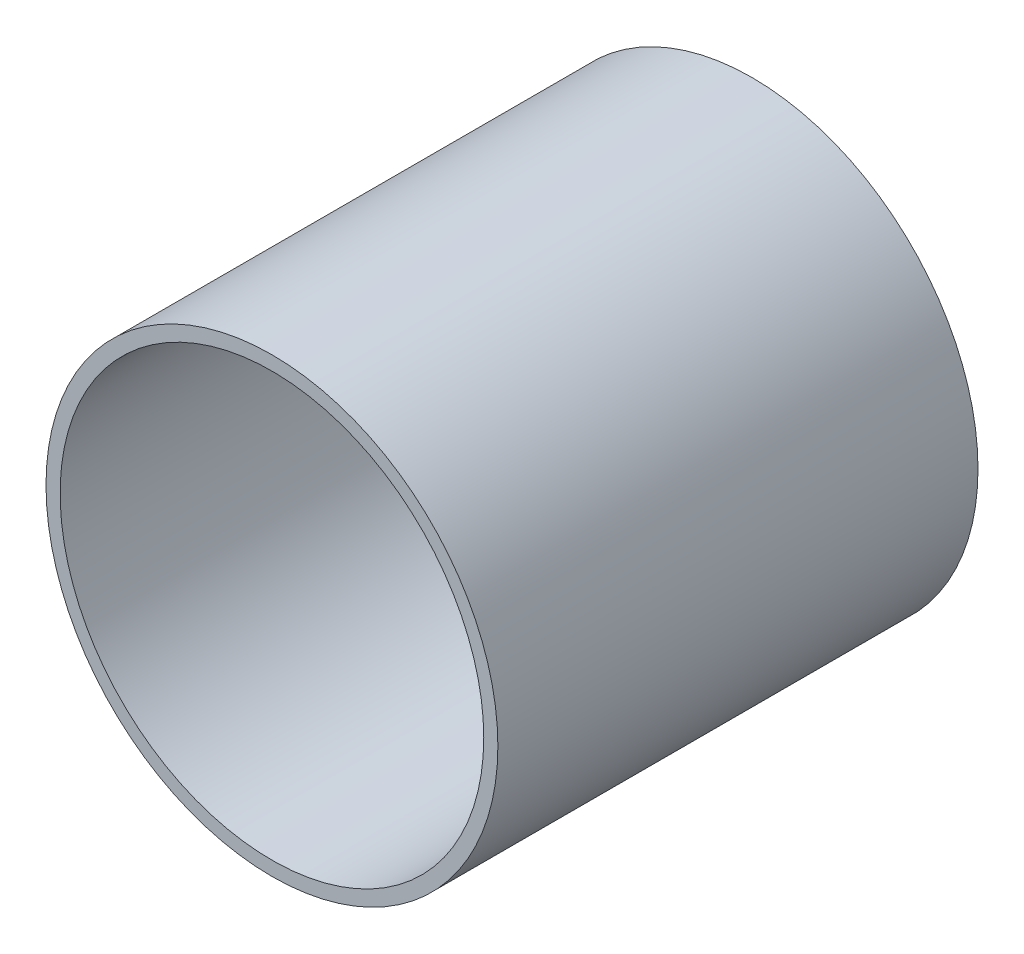
from build123d import *

# Parameters (mm, degrees)
SKETCH_1_R      = 80
SKETCH_1_R_2    = 75
EXTRUDE_1_DEPTH = 170


with BuildPart() as part:
    # 草图1 → 凸台-拉伸1 (new body)
    with BuildSketch(Plane.XY):
        Circle(SKETCH_1_R)
        Circle(SKETCH_1_R_2, mode=Mode.SUBTRACT)
    extrude(amount=EXTRUDE_1_DEPTH)


solid = part.part
